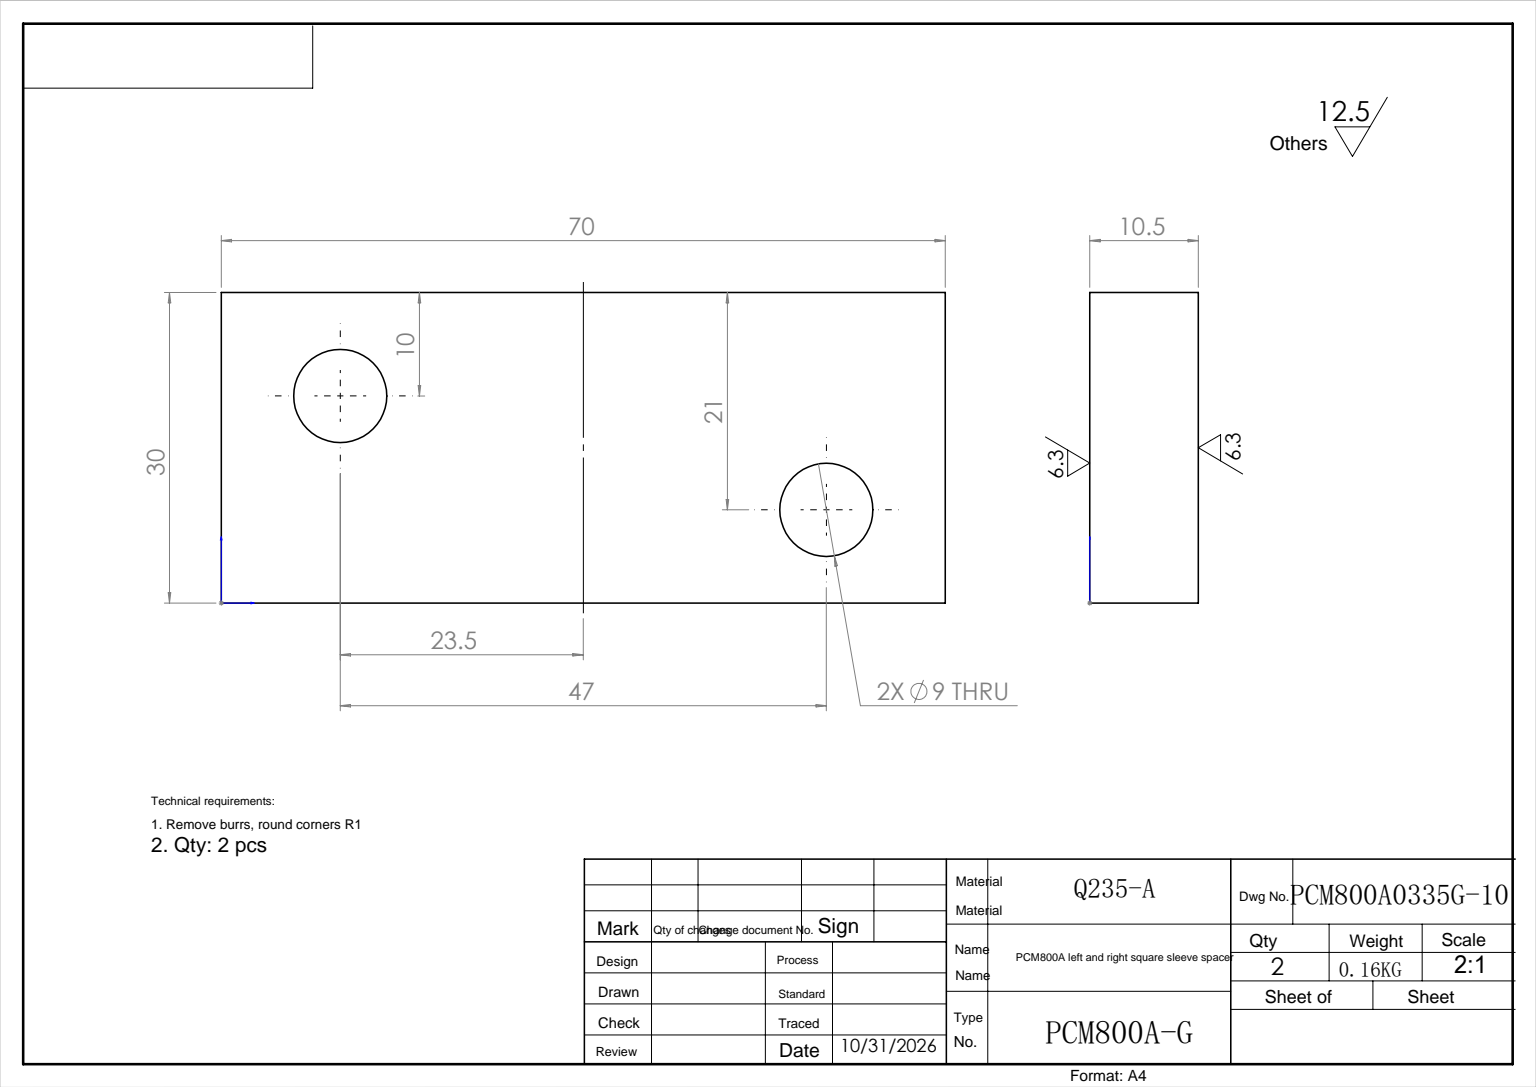
SolidWorks part; units mm, degrees
ref_plane "前视基准面" through (0, 0, 0) normal (0, 0, 1) x (1, 0, 0)
ref_plane "上视基准面" through (0, 0, 0) normal (0, 1, 0) x (1, 0, 0)
ref_plane "右视基准面" through (0, 0, 0) normal (1, 0, 0) x (0, 0, -1)
sketch "草图1" plane through (0, 0, 0) normal (0, 0, 1) x (1, 0, 0)
  line L0 (35, 30) -> (35, -37.8291) construction
  line L1 (0, 0) -> (70, 0)
  line L2 (0, 0) -> (0, 30)
  line L3 (0, 30) -> (70, 30)
  line L4 (70, 0) -> (70, 30)
  circle A0 centre (11.5, 20) radius 4.5
  circle A1 centre (58.5, 9) radius 4.5
  dimension "D7" = 9
  dimension "D8" = 9
  dimension "D1" = 30
  dimension "D2" = 70
  dimension "D3" = 23.5
  dimension "D4" = 23.5
  dimension "D5" = 10
  dimension "D6" = 21
extrude "凸台-拉伸1" add sketch "草图1" along normal blind 10.5
